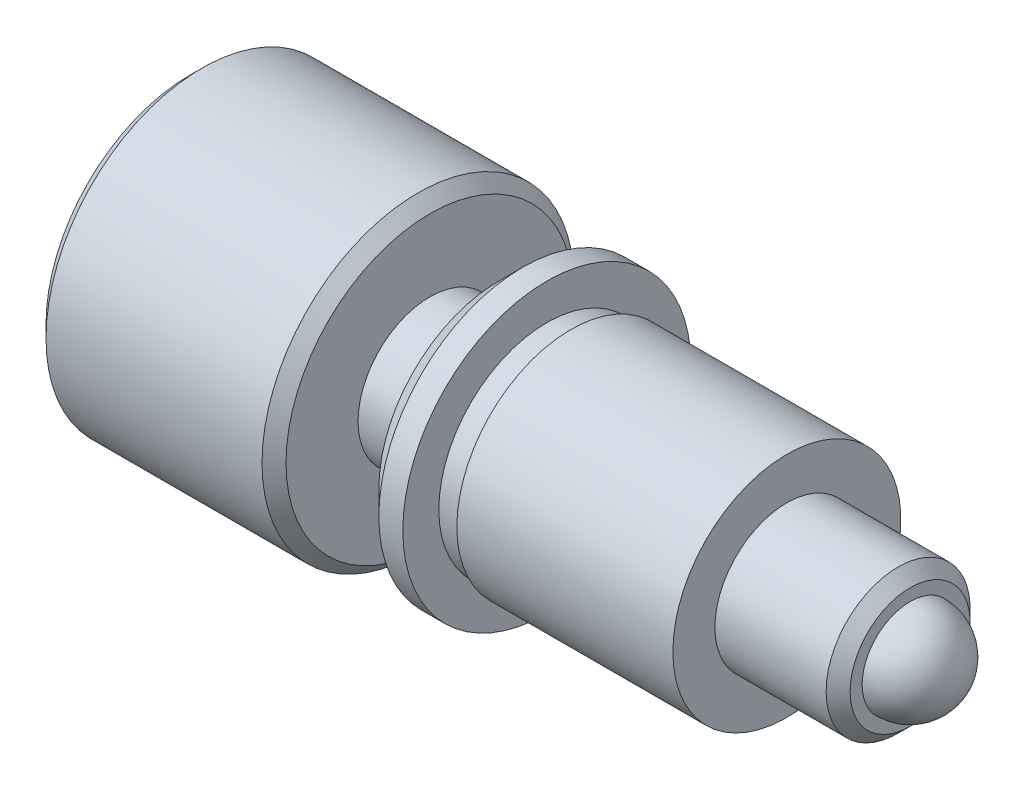
from build123d import *


with BuildPart() as part:
    # Sketch1 → Revolve1 (revolve)
    with BuildSketch(Plane(origin=(0, 0, 0), x_dir=(1, 0, 0), z_dir=(0, 1, 0)), mode=Mode.PRIVATE) as revolve1_sk:
        with BuildLine():
            Line((-15.545938878, 0), (-15.545938878, 6))
            Line((-15.545938878, 6), (-15.045938878, 6.5))
            Line((-15.045938878, 6.5), (-6.045938878, 6.5))
            Line((-6.045938878, 6.5), (-5.545938878, 6))
            Line((-5.545938878, 6), (-5.545938878, 3))
            Line((-5.545938878, 3), (-2.680089485, 3))
            Line((-2.680089485, 3), (-2.680089485, 5))
            Line((-2.680089485, 5), (-1.680089485, 6))
            Line((-1.680089485, 6), (-0.680089485, 6))
            Line((-0.680089485, 6), (-0.680089485, 4.5))
            Line((-0.680089485, 4.5), (0.319910515, 4.5))
            Line((0.319910515, 4.5), (0.319910515, 4.75))
            Line((0.319910515, 4.75), (9.319910515, 4.75))
            Line((9.319910515, 4.75), (9.319910515, 3))
            Line((9.319910515, 3), (13.954061122, 3))
            Line((13.954061122, 3), (14.454061122, 2.5))
            Line((14.454061122, 2.5), (14.454061122, 2))
            ThreePointArc((14.454061122, 2), (15.868274684, 1.414213562), (16.454061122, 0))
            Line((16.454061122, 0), (-15.545938878, 0))
        make_face()
    revolve(revolve1_sk.sketch.rotate(Axis((-122.432679922, 0, 0), (1, 0, 0)), 180), axis=Axis((-122.432679922, 0, 0), (1, 0, 0)))


solid = part.part
